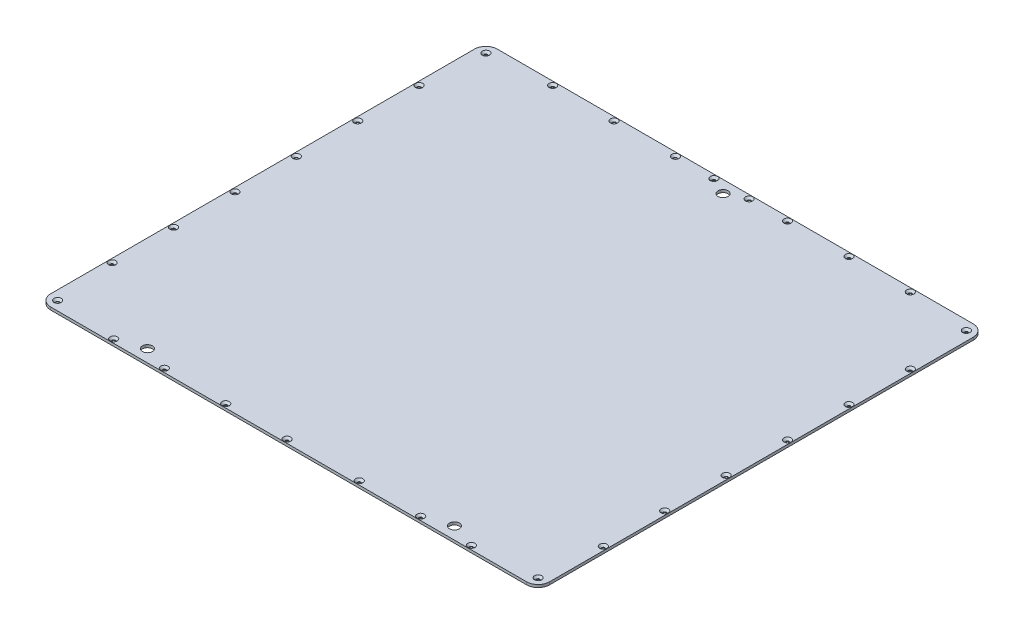
SolidWorks part; units mm, degrees
ref_plane "Front Plane" through (0, 0, 0) normal (0, 0, 1) x (1, 0, 0)
ref_plane "Top Plane" through (0, 0, 0) normal (0, 1, 0) x (1, 0, 0)
ref_plane "Right Plane" through (0, 0, 0) normal (1, 0, 0) x (0, 0, -1)
sketch "Sketch1" plane through (0, 0, 0) normal (0, 1, 0) x (1, 0, 0)
  line L1 (-310, -291) -> (310, -291)
  line L2 (-325, -276) -> (-325, 276)
  line L3 (-310, 291) -> (310, 291)
  line L4 (325, -276) -> (325, 276)
  line L5 (-325, -291) -> (325, 291) construction
  line L6 (-325, 291) -> (325, -291) construction
  arc A0 (-310, -291) -> (-325, -276) centre (-310, -276) cw
  arc A1 (310, -291) -> (325, -276) centre (310, -276) ccw
  arc A2 (310, 291) -> (325, 276) centre (310, 276) cw
  arc A3 (-325, 276) -> (-310, 291) centre (-310, 276) cw
  point P0 (0, 0)
  dimension "D3" = 15
  dimension "D1" = 650
  dimension "D2" = 582
extrude "Boss-Extrude1" add sketch "Sketch1" along normal blind 3.5
sketch "Sketch2" plane through (0, 3.5, 0) normal (0, 1, 0) x (1, 0, 0)
  line L0 (-325, 276) -> (-325, -276) construction
  line L1 (310, 291) -> (-310, 291) construction
  line L2 (-310, -291) -> (310, -291) construction
  line L3 (325, -276) -> (325, 276) construction
  circle A0 centre (0, 275) radius 6.5
  circle A1 centre (200, -275) radius 6.5
  circle A2 centre (-200, -275) radius 6.5
  dimension "D1" = 13
  dimension "D2" = 13
  dimension "D3" = 13
  dimension "D4" = 325
  dimension "D5" = 16
  dimension "D6" = 16
  dimension "D7" = 16
  dimension "D8" = 125
  dimension "D9" = 125
extrude "Cut-Extrude1" cut sketch "Sketch2" against normal through all
hole_wizard "CSK for M4 Flat Head Machine Screw1" positions "Sketch3" profile "Sketch4" countersink size "M4" standard "ANSI Metric"
sketch "Sketch3" plane through (0, 3.5, 0) normal (0, 1, 0) x (1, 0, 0)
  line L0 (310, 291) -> (-310, 291) construction
  line L1 (-325, 276) -> (-325, -276) construction
  line L4 (325, -276) -> (325, 276) construction
  line L5 (-310, -291) -> (310, -291) construction
  point P2 (-233, 286)
  point P7 (-313, 279)
  point P9 (-153, 286)
  point P11 (-73, 286)
  point P13 (-23, 286)
  point P21 (73, 286)
  point P23 (153, 286)
  point P25 (313, 279)
  point P27 (-320, 199)
  point P29 (-320, 119)
  point P31 (-320, 39)
  point P33 (-320, -41)
  point P35 (-320, -121)
  point P37 (-320, -201)
  point P39 (-313, -279)
  point P41 (-233, -286)
  point P43 (-167, -286)
  point P45 (-87, -286)
  point P47 (-7, -286)
  point P49 (87, -286)
  point P51 (167, -286)
  point P53 (313, -279)
  point P55 (320, -201)
  point P57 (320, -121)
  point P59 (320, -41)
  point P61 (320, 39)
  point P63 (320, 119)
  point P65 (320, 199)
  point P72 (233, 286)
  point P84 (23, 286)
  point P89 (233, -286)
  dimension "D1" = 5
  dimension "D2" = 12
  dimension "D3" = 12
  dimension "D4" = 80
  dimension "D5" = 80
  dimension "D6" = 80
  dimension "D7" = 50
  dimension "D8" = 5
  dimension "D9" = 12
  dimension "D10" = 50
  dimension "D11" = 5
  dimension "D12" = 80
  dimension "D13" = 80
  dimension "D14" = 80
  dimension "D15" = 12
  dimension "D16" = 80
  dimension "D17" = 80
  dimension "D18" = 80
  dimension "D19" = 80
  dimension "D20" = 80
  dimension "D21" = 80
  dimension "D22" = 12
  dimension "D23" = 12
  dimension "D24" = 5
  dimension "D25" = 80
  dimension "D26" = 80
  dimension "D27" = 80
  dimension "D28" = 80
  dimension "D29" = 80
  dimension "D30" = 80
  dimension "D31" = 12
  dimension "D32" = 12
  dimension "D33" = 80
  dimension "D34" = 80
  dimension "D35" = 66
  dimension "D36" = 80
  dimension "D37" = 5
  dimension "D38" = 80
  dimension "D39" = 66
  dimension "D40" = 80
sketch "Sketch4" plane through (-233, 3.5, -286) normal (1, 0, 0) x (0, 0, 1)
  line L0 (0, 0) -> (0, 8.7919)
  line L1 (0, 8.7919) -> (2.15, 7.5)
  line L2 (2.15, 7.5) -> (2.15, 2.55)
  line L3 (2.15, 2.55) -> (4.7, 0)
  line L5 (4.7, 0) -> (0, 0)
  line L6 (-2.15, 2.55) -> (-4.7, 0) construction
  line L10 (0, 8.7919) -> (-2.15, 7.5) construction
  line L11 (0, -6.35) -> (0, 107.95) construction
  dimension "孔直径" = 4.3
  dimension "孔深度" = 7.5
  dimension "近端锥形沉头孔直径" = 9.4
  dimension "近端锥形沉头孔角度" = 90
  dimension "导头角度" = 118
